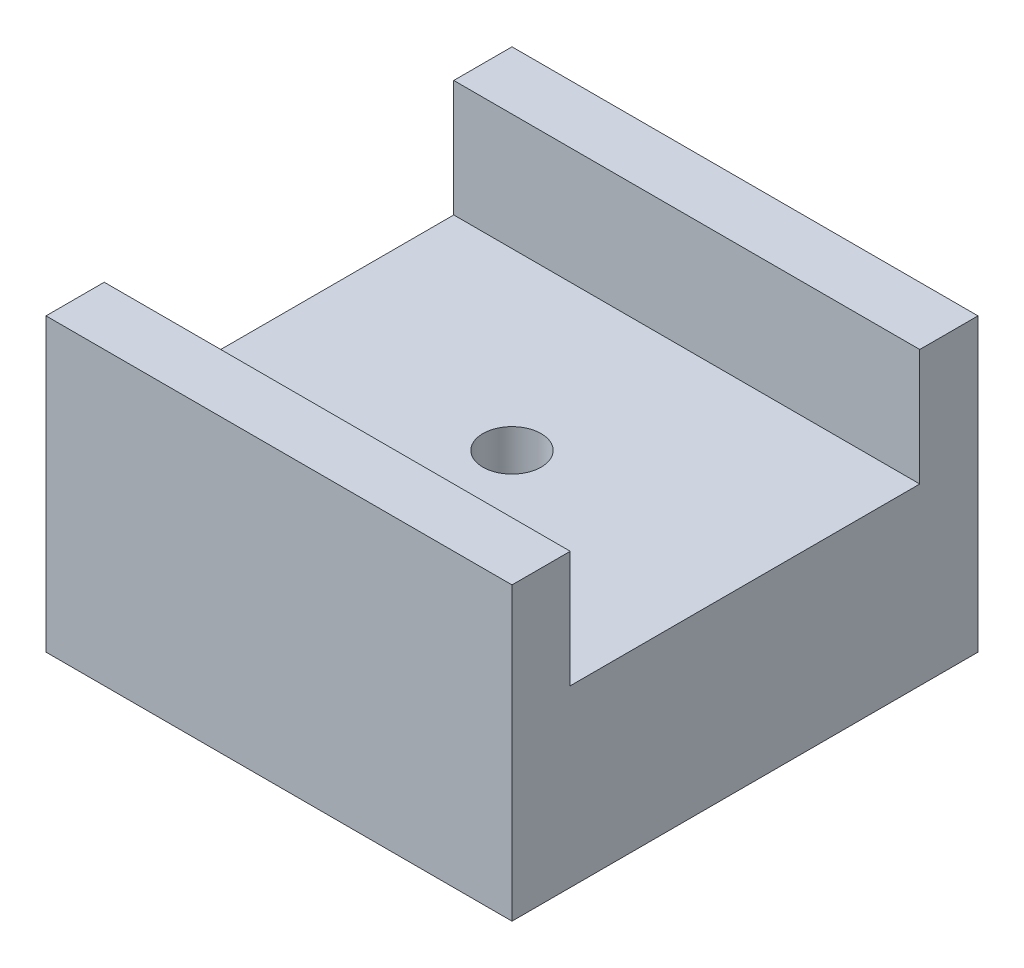
SolidWorks part; units mm, degrees
ref_plane "Front Plane" through (0, 0, 0) normal (0, 0, 1) x (1, 0, 0)
ref_plane "Top Plane" through (0, 0, 0) normal (0, 1, 0) x (1, 0, 0)
ref_plane "Right Plane" through (0, 0, 0) normal (1, 0, 0) x (0, 0, -1)
sketch "Sketch1" plane through (0, 0, 0) normal (0, 1, 0) x (1, 0, 0)
  line L1 (-20, 20) -> (20, 20)
  line L2 (-20, 20) -> (-20, -20)
  line L3 (-20, -20) -> (20, -20)
  line L4 (20, 20) -> (20, -20)
  line L5 (-20, 20) -> (20, -20) construction
  line L6 (-20, -20) -> (20, 20) construction
  point P0 (0, 0)
  dimension "D1" = 40
  dimension "D2" = 40
extrude "Boss-Extrude1" add sketch "Sketch1" along normal blind 25
sketch "Sketch2" plane through (0, 25, 0) normal (0, 1, 0) x (1, 0, 0)
  line L0 (20, -20) -> (20, 20) construction
  line L1 (-20, -15) -> (20, -15)
  line L2 (-20, -15) -> (-20, 15)
  line L3 (-20, 15) -> (20, 15)
  line L4 (20, -15) -> (20, 15)
  line L5 (-20, -15) -> (20, 15) construction
  line L6 (-20, 15) -> (20, -15) construction
  point P0 (0, 0)
  dimension "D1" = 30
extrude "Cut-Extrude1" cut sketch "Sketch2" against normal blind 10
hole_wizard "M6 Tapped Hole1" positions "Sketch3" profile "Sketch4" tap size "M6" standard "ISO" end condition through all
sketch "Sketch3" plane through (0, 0, 0) normal (0, -1, 0) x (-1, 0, 0)
  point P0 (0, 0)
sketch "Sketch4" plane through (0, 0, 0) normal (1, 0, 0) x (0, 0, -1)
  line L0 (0, 0) -> (0, 25)
  line L1 (0, 25) -> (2.5, 25)
  line L2 (2.5, 25) -> (2.5, 0)
  line L5 (2.5, 0) -> (0, 0)
  line L11 (0, -6.35) -> (0, 107.95) construction
  dimension "通孔螺纹孔钻头直径" = 5
  dimension "通孔螺纹孔钻头深度" = 25
cosmetic thread "Hole Thread1" parameters "D2"=6
